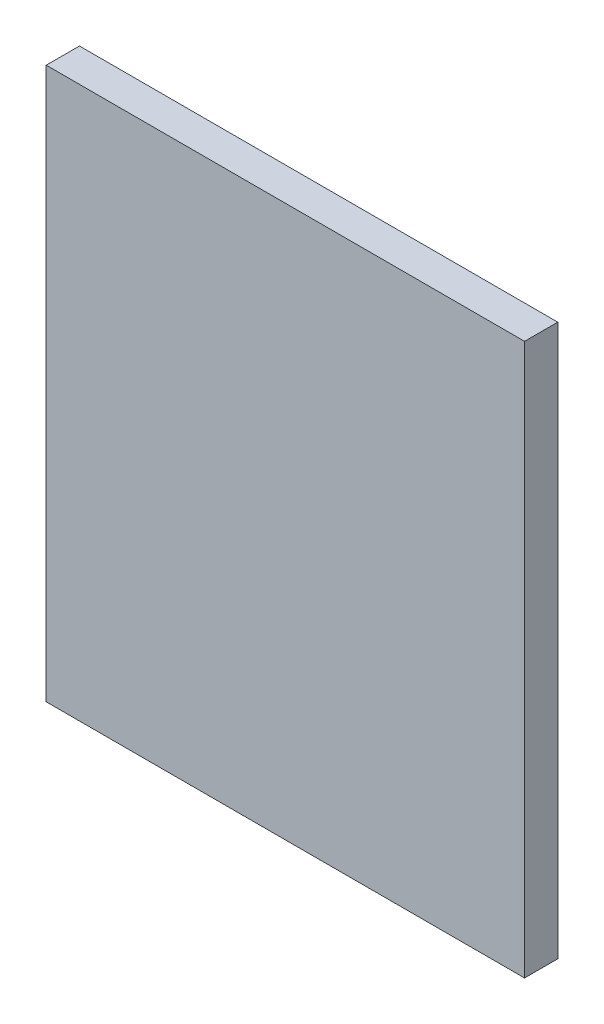
SolidWorks part; units mm, degrees
ref_plane "Front Plane" through (0, 0, 0) normal (0, 0, 1) x (1, 0, 0)
ref_plane "Top Plane" through (0, 0, 0) normal (0, 1, 0) x (1, 0, 0)
ref_plane "Right Plane" through (0, 0, 0) normal (1, 0, 0) x (0, 0, -1)
sketch "Sketch1" plane through (0, 0, 0) normal (0, 0, 1) x (1, 0, 0)
  line L1 (0, 0) -> (360, 0)
  line L2 (0, 0) -> (0, -415)
  line L3 (0, -415) -> (360, -415)
  line L4 (360, 0) -> (360, -415)
  dimension "D1" = 360
  dimension "D2" = 415
extrude "Boss-Extrude1" add sketch "Sketch1" along normal blind 25
